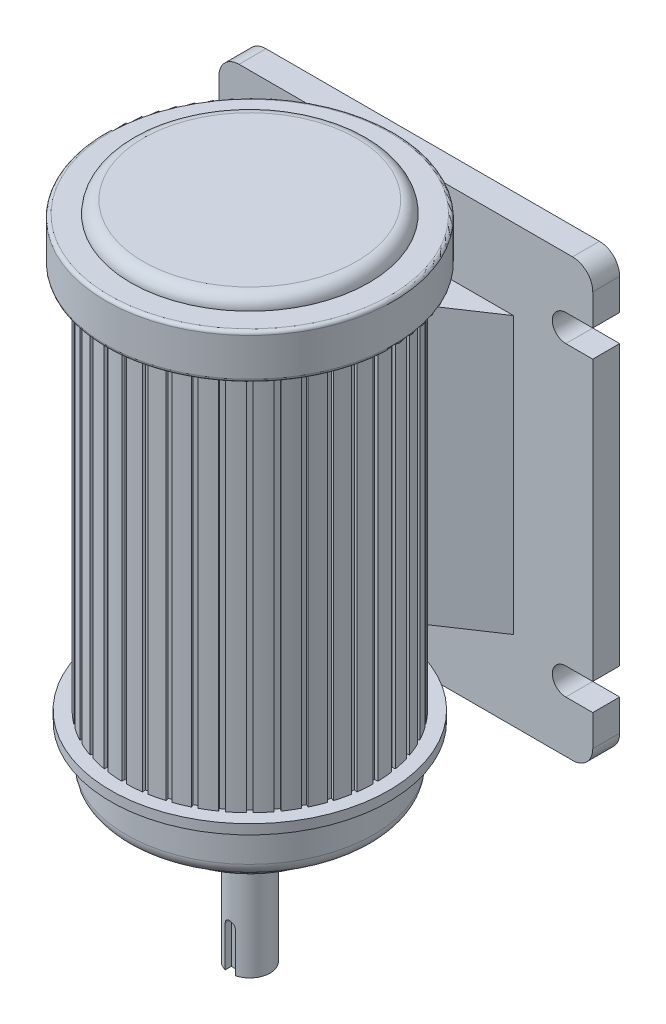
SolidWorks part; units mm, degrees
ref_plane "Front Plane" through (0, 0, 0) normal (0, 0, 1) x (1, 0, 0)
ref_plane "Top Plane" through (0, 0, 0) normal (0, 1, 0) x (1, 0, 0)
ref_plane "Right Plane" through (0, 0, 0) normal (1, 0, 0) x (0, 0, -1)
other "Configuration Table"
sketch "Sketch1" plane through (0, 0, 0) normal (0, 0, 1) x (1, 0, 0)
  line L5 (-18.5243, 142.4072) -> (36.9765, 142.4072)
  line L6 (-18.5243, 142.4072) -> (-18.5243, 77.6701)
  line L7 (-18.5243, 77.6701) -> (36.9765, 77.6701)
  line L12 (36.9765, 142.4072) -> (36.9765, 77.6701)
  line L13 (-18.5243, 142.4072) -> (36.9765, 77.6701) construction
  line L14 (-18.5243, 77.6701) -> (36.9765, 142.4072) construction
  point P2 (9.2261, 110.0386)
extrude "Boss-Extrude1" add sketch "Sketch1" along normal blind 4
sketch "Sketch2" plane through (0, 0, 4) normal (0, 0, 1) x (1, 0, 0)
  line L0 (-14.5271, 134.7549) -> (-18.5243, 134.7549)
  line L1 (-14.5271, 130.7549) -> (-18.5243, 130.7549)
  line L2 (-18.5243, 89.3223) -> (-18.5243, 85.3223)
  line L3 (36.9765, 130.7549) -> (36.9765, 134.7549)
  line L4 (36.9765, 77.6701) -> (36.9765, 142.4072)
  line L5 (36.9765, 142.4072) -> (-18.5243, 142.4072)
  line L6 (-18.5243, 142.4072) -> (-18.5243, 77.6701)
  line L7 (-18.5243, 77.6701) -> (36.9765, 77.6701)
  line L8 (36.9765, 85.3223) -> (36.9765, 89.3223)
  line L10 (-18.5243, 134.7549) -> (-18.5243, 130.7549)
  line L12 (32.9793, 130.7549) -> (36.9765, 130.7549)
  line L13 (32.9793, 134.7549) -> (36.9765, 134.7549)
  line L14 (32.9793, 85.3223) -> (36.9765, 85.3223)
  line L15 (32.9793, 89.3223) -> (36.9765, 89.3223)
  line L16 (-14.5271, 89.3223) -> (-18.5243, 89.3223)
  line L17 (-14.5271, 85.3223) -> (-18.5243, 85.3223)
  arc A0 (-14.5271, 130.7549) -> (-14.5271, 134.7549) centre (-14.5271, 132.7549) ccw
  arc A1 (32.9793, 130.7549) -> (32.9793, 134.7549) centre (32.9793, 132.7549) cw
  arc A2 (32.9793, 89.3223) -> (32.9793, 85.3223) centre (32.9793, 87.3223) ccw
  arc A3 (-14.5271, 89.3223) -> (-14.5271, 85.3223) centre (-14.5271, 87.3223) cw
  dimension "D1" = 0
extrude "Cut-Extrude1" cut sketch "Sketch2" against normal blind 4
fillet "Fillet1" radius 3 4 edges at (36.9765, 142.4072, 2) (-18.5243, 142.4072, 2) (-18.5243, 77.6701, 2) (36.9765, 77.6701, 2)
sketch "Sketch3" plane through (9.2261, -4.2483, 39.612) normal (1, 0, 0) x (0, 1, 0)
  line L0 (114.2869, -35.612) -> (114.2869, 7.7128) construction
  line L1 (93.5706, -35.612) -> (135.0032, -35.612) construction
  line L3 (75.2706, -12.4595) -> (153.1789, -12.4595)
  line L4 (75.2706, -12.4595) -> (75.2706, -0.1704)
  line L5 (87.5845, 6.1907) -> (144.7264, 6.1907)
  line L6 (153.1789, -12.4595) -> (153.1789, 3.3865)
  line L7 (151.3529, 5.2125) -> (151.3529, 8.4086)
  line L8 (150.8529, 8.9086) -> (145.2264, 8.9086)
  line L9 (144.7264, 8.4086) -> (144.7264, 6.1907)
  line L10 (87.5845, 6.1907) -> (87.5845, 8.1927)
  line L11 (87.5845, 8.1927) -> (86.1419, 8.1927)
  line L12 (86.1419, 8.1927) -> (86.1419, 7.166)
  line L13 (86.1419, 7.166) -> (86.1419, 5.8831)
  line L14 (86.1419, 5.8831) -> (80.7228, 5.8831)
  line L15 (78.7228, 3.8831) -> (78.7228, -0.0402)
  line L16 (78.7228, -0.0402) -> (77.8437, -0.6822)
  line L17 (77.8437, -0.6822) -> (77.8437, 0.7371)
  line L18 (77.6437, 0.9371) -> (76.7521, 0.9371)
  line L19 (76.5521, 0.7371) -> (76.5521, 0.0296)
  line L20 (76.5521, 0.0296) -> (75.4706, 0.0296)
  arc A0 (153.1789, 3.3865) -> (151.3529, 5.2125) centre (151.3529, 3.3865) ccw
  arc A1 (145.2264, 8.9086) -> (144.7264, 8.4086) centre (145.2264, 8.4086) ccw
  arc A2 (151.3529, 8.4086) -> (150.8529, 8.9086) centre (150.8529, 8.4086) ccw
  arc A3 (80.7228, 5.8831) -> (78.7228, 3.8831) centre (80.7228, 3.8831) ccw
  arc A4 (76.7521, 0.9371) -> (76.5521, 0.7371) centre (76.7521, 0.7371) ccw
  arc A5 (77.8437, 0.7371) -> (77.6437, 0.9371) centre (77.6437, 0.7371) ccw
  arc A6 (75.4706, 0.0296) -> (75.2706, -0.1704) centre (75.4706, -0.1704) ccw
  dimension "D1" = 0.5
  dimension "D2" = 2
  dimension "D3" = 0.2
  dimension "D4" = 0.2
revolve "Revolve1" add sketch "Sketch3" angle 360 about L3
ref_plane "Plane1" through (0, 109.9765, 0) normal (0, 1, 0) x (1, 0, 0)
sketch "Sketch5" plane through (0, 83.3362, 0) normal (0, 1, 0) x (1, 0, 0)
  line L0 (11.7885, -8.6793) -> (11.7149, -9.1436)
  line L6 (8.8671, -8.5059) -> (8.8671, -8.976)
  line L7 (8.8671, -8.976) -> (9.5851, -8.976)
  line L8 (9.5851, -8.5059) -> (9.5851, -8.976)
  line L9 (9.2261, -8.5024) -> (9.5851, -8.976) construction
  line L10 (8.8671, -8.976) -> (9.2261, -8.5024) construction
  line L11 (11.7149, -9.1436) -> (12.4241, -9.2559)
  line L12 (12.4977, -8.7916) -> (12.4241, -9.2559)
  line L13 (12.1436, -8.732) -> (12.4241, -9.2559) construction
  line L14 (11.7149, -9.1436) -> (12.1436, -8.732) construction
  line L15 (14.6468, -9.3075) -> (14.5015, -9.7546)
  line L16 (14.5015, -9.7546) -> (15.1844, -9.9765)
  line L17 (15.3297, -9.5294) -> (15.1844, -9.9765)
  line L18 (14.9893, -9.4152) -> (15.1844, -9.9765) construction
  line L19 (14.5015, -9.7546) -> (14.9893, -9.4152) construction
  line L20 (17.3716, -10.3752) -> (17.1582, -10.7941)
  line L21 (17.1582, -10.7941) -> (17.798, -11.1201)
  line L22 (18.0114, -10.7012) -> (17.798, -11.1201)
  line L23 (17.6931, -10.5351) -> (17.798, -11.1201) construction
  line L24 (17.1582, -10.7941) -> (17.6931, -10.5351) construction
  line L25 (19.8959, -11.856) -> (19.6196, -12.2364)
  line L26 (19.6196, -12.2364) -> (20.2005, -12.6584)
  line L27 (20.4768, -12.2781) -> (20.2005, -12.6584)
  line L28 (20.1884, -12.0643) -> (20.2005, -12.6584) construction
  line L29 (19.6196, -12.2364) -> (20.1884, -12.0643) construction
  line L30 (22.1574, -13.7135) -> (21.825, -14.0459)
  line L31 (21.825, -14.0459) -> (22.3327, -14.5536)
  line L32 (22.6652, -14.2212) -> (22.3327, -14.5536)
  line L33 (22.4137, -13.9649) -> (22.3327, -14.5536) construction
  line L34 (21.825, -14.0459) -> (22.4137, -13.9649) construction
  line L35 (24.1006, -15.9018) -> (23.7202, -16.1782)
  line L36 (23.7202, -16.1782) -> (24.1423, -16.7591)
  line L37 (24.5226, -16.4827) -> (24.1423, -16.7591)
  line L38 (24.3144, -16.1903) -> (24.1423, -16.7591) construction
  line L39 (23.7202, -16.1782) -> (24.3144, -16.1903) construction
  line L40 (25.6774, -18.3672) -> (25.2586, -18.5807)
  line L41 (25.2586, -18.5807) -> (25.5845, -19.2204)
  line L42 (26.0034, -19.007) -> (25.5845, -19.2204)
  line L43 (25.8435, -18.6856) -> (25.5845, -19.2204) construction
  line L44 (25.2586, -18.5807) -> (25.8435, -18.6856) construction
  line L45 (26.8492, -21.049) -> (26.4021, -21.1942)
  line L46 (26.4021, -21.1942) -> (26.624, -21.8771)
  line L47 (27.0711, -21.7319) -> (26.624, -21.8771)
  line L48 (26.9634, -21.3893) -> (26.624, -21.8771) construction
  line L49 (26.4021, -21.1942) -> (26.9634, -21.3893) construction
  line L50 (27.587, -23.881) -> (27.1227, -23.9545)
  line L51 (27.1227, -23.9545) -> (27.2351, -24.6637)
  line L52 (27.6994, -24.5902) -> (27.2351, -24.6637)
  line L53 (27.6466, -24.235) -> (27.2351, -24.6637) construction
  line L54 (27.1227, -23.9545) -> (27.6466, -24.235) construction
  line L55 (27.8728, -26.7935) -> (27.4027, -26.7935)
  line L56 (27.4027, -26.7935) -> (27.4027, -27.5116)
  line L57 (27.8728, -27.5116) -> (27.4027, -27.5116)
  line L58 (27.8762, -27.1526) -> (27.4027, -27.5116) construction
  line L59 (27.4027, -26.7935) -> (27.8762, -27.1526) construction
  line L60 (27.6994, -29.7149) -> (27.2351, -29.6414)
  line L61 (27.2351, -29.6414) -> (27.1227, -30.3506)
  line L62 (27.587, -30.4241) -> (27.1227, -30.3506)
  line L63 (27.6466, -30.0701) -> (27.1227, -30.3506) construction
  line L64 (27.2351, -29.6414) -> (27.6466, -30.0701) construction
  line L65 (27.0711, -32.5733) -> (26.624, -32.428)
  line L66 (26.624, -32.428) -> (26.4021, -33.1109)
  line L67 (26.8492, -33.2561) -> (26.4021, -33.1109)
  line L68 (26.9634, -32.9158) -> (26.4021, -33.1109) construction
  line L69 (26.624, -32.428) -> (26.9634, -32.9158) construction
  line L70 (26.0034, -35.2981) -> (25.5845, -35.0847)
  line L71 (25.5845, -35.0847) -> (25.2586, -35.7244)
  line L72 (25.6774, -35.9379) -> (25.2586, -35.7244)
  line L73 (25.8435, -35.6195) -> (25.2586, -35.7244) construction
  line L74 (25.5845, -35.0847) -> (25.8435, -35.6195) construction
  line L75 (24.5226, -37.8224) -> (24.1423, -37.546)
  line L76 (24.1423, -37.546) -> (23.7202, -38.1269)
  line L77 (24.1006, -38.4033) -> (23.7202, -38.1269)
  line L78 (24.3144, -38.1148) -> (23.7202, -38.1269) construction
  line L79 (24.1423, -37.546) -> (24.3144, -38.1148) construction
  line L80 (22.6652, -40.0839) -> (22.3327, -39.7515)
  line L81 (22.3327, -39.7515) -> (21.825, -40.2592)
  line L82 (22.1574, -40.5916) -> (21.825, -40.2592)
  line L83 (22.4137, -40.3402) -> (21.825, -40.2592) construction
  line L84 (22.3327, -39.7515) -> (22.4137, -40.3402) construction
  line L85 (20.4768, -42.027) -> (20.2005, -41.6467)
  line L86 (20.2005, -41.6467) -> (19.6196, -42.0688)
  line L87 (19.8959, -42.4491) -> (19.6196, -42.0688)
  line L88 (20.1884, -42.2408) -> (19.6196, -42.0688) construction
  line L89 (20.2005, -41.6467) -> (20.1884, -42.2408) construction
  line L90 (18.0114, -43.6039) -> (17.798, -43.185)
  line L91 (17.798, -43.185) -> (17.1582, -43.511)
  line L92 (17.3716, -43.9299) -> (17.1582, -43.511)
  line L93 (17.6931, -43.77) -> (17.1582, -43.511) construction
  line L94 (17.798, -43.185) -> (17.6931, -43.77) construction
  line L95 (15.3297, -44.7757) -> (15.1844, -44.3286)
  line L96 (15.1844, -44.3286) -> (14.5015, -44.5505)
  line L97 (14.6468, -44.9976) -> (14.5015, -44.5505)
  line L98 (14.9893, -44.8899) -> (14.5015, -44.5505) construction
  line L99 (15.1844, -44.3286) -> (14.9893, -44.8899) construction
  line L100 (12.4977, -45.5135) -> (12.4241, -45.0492)
  line L101 (12.4241, -45.0492) -> (11.7149, -45.1615)
  line L102 (11.7885, -45.6258) -> (11.7149, -45.1615)
  line L103 (12.1436, -45.5731) -> (11.7149, -45.1615) construction
  line L104 (12.4241, -45.0492) -> (12.1436, -45.5731) construction
  line L105 (9.5851, -45.7992) -> (9.5851, -45.3292)
  line L106 (9.5851, -45.3292) -> (8.8671, -45.3292)
  line L107 (8.8671, -45.7992) -> (8.8671, -45.3292)
  line L108 (9.2261, -45.8027) -> (8.8671, -45.3292) construction
  line L109 (9.5851, -45.3292) -> (9.2261, -45.8027) construction
  line L110 (6.6637, -45.6258) -> (6.7372, -45.1615)
  line L111 (6.7372, -45.1615) -> (6.028, -45.0492)
  line L112 (5.9545, -45.5135) -> (6.028, -45.0492)
  line L113 (6.3086, -45.5731) -> (6.028, -45.0492) construction
  line L114 (6.7372, -45.1615) -> (6.3086, -45.5731) construction
  line L115 (3.8054, -44.9976) -> (3.9506, -44.5505)
  line L116 (3.9506, -44.5505) -> (3.2678, -44.3286)
  line L117 (3.1225, -44.7757) -> (3.2678, -44.3286)
  line L118 (3.4629, -44.8899) -> (3.2678, -44.3286) construction
  line L119 (3.9506, -44.5505) -> (3.4629, -44.8899) construction
  line L120 (1.0805, -43.9299) -> (1.294, -43.511)
  line L121 (1.294, -43.511) -> (0.6542, -43.185)
  line L122 (0.4408, -43.6039) -> (0.6542, -43.185)
  line L123 (0.7591, -43.77) -> (0.6542, -43.185) construction
  line L124 (1.294, -43.511) -> (0.7591, -43.77) construction
  line L125 (-1.4437, -42.4491) -> (-1.1674, -42.0688)
  line L126 (-1.1674, -42.0688) -> (-1.7483, -41.6467)
  line L127 (-2.0246, -42.027) -> (-1.7483, -41.6467)
  line L128 (-1.7362, -42.2408) -> (-1.7483, -41.6467) construction
  line L129 (-1.1674, -42.0688) -> (-1.7362, -42.2408) construction
  line L130 (-3.7053, -40.5916) -> (-3.3729, -40.2592)
  line L131 (-3.3729, -40.2592) -> (-3.8806, -39.7515)
  line L132 (-4.213, -40.0839) -> (-3.8806, -39.7515)
  line L133 (-3.9616, -40.3402) -> (-3.8806, -39.7515) construction
  line L134 (-3.3729, -40.2592) -> (-3.9616, -40.3402) construction
  line L135 (-5.6484, -38.4033) -> (-5.2681, -38.1269)
  line L136 (-5.2681, -38.1269) -> (-5.6901, -37.546)
  line L137 (-6.0704, -37.8224) -> (-5.6901, -37.546)
  line L138 (-5.8622, -38.1148) -> (-5.6901, -37.546) construction
  line L139 (-5.2681, -38.1269) -> (-5.8622, -38.1148) construction
  line L140 (-7.2253, -35.9379) -> (-6.8064, -35.7244)
  line L141 (-6.8064, -35.7244) -> (-7.1324, -35.0847)
  line L142 (-7.5512, -35.2981) -> (-7.1324, -35.0847)
  line L143 (-7.3913, -35.6195) -> (-7.1324, -35.0847) construction
  line L144 (-6.8064, -35.7244) -> (-7.3913, -35.6195) construction
  line L145 (-8.397, -33.2561) -> (-7.9499, -33.1109)
  line L146 (-7.9499, -33.1109) -> (-8.1718, -32.428)
  line L147 (-8.6189, -32.5733) -> (-8.1718, -32.428)
  line L148 (-8.5113, -32.9158) -> (-8.1718, -32.428) construction
  line L149 (-7.9499, -33.1109) -> (-8.5113, -32.9158) construction
  line L150 (-9.1349, -30.4241) -> (-8.6706, -30.3506)
  line L151 (-8.6706, -30.3506) -> (-8.7829, -29.6414)
  line L152 (-9.2472, -29.7149) -> (-8.7829, -29.6414)
  line L153 (-9.1945, -30.0701) -> (-8.7829, -29.6414) construction
  line L154 (-8.6706, -30.3506) -> (-9.1945, -30.0701) construction
  line L155 (-9.4206, -27.5116) -> (-8.9505, -27.5116)
  line L156 (-8.9505, -27.5116) -> (-8.9505, -26.7935)
  line L157 (-9.4206, -26.7935) -> (-8.9505, -26.7935)
  line L158 (-9.4241, -27.1526) -> (-8.9505, -26.7935) construction
  line L159 (-8.9505, -27.5116) -> (-9.4241, -27.1526) construction
  line L160 (-9.2472, -24.5902) -> (-8.7829, -24.6637)
  line L161 (-8.7829, -24.6637) -> (-8.6706, -23.9545)
  line L162 (-9.1349, -23.881) -> (-8.6706, -23.9545)
  line L163 (-9.1945, -24.235) -> (-8.6706, -23.9545) construction
  line L164 (-8.7829, -24.6637) -> (-9.1945, -24.235) construction
  line L165 (-8.6189, -21.7319) -> (-8.1718, -21.8771)
  line L166 (-8.1718, -21.8771) -> (-7.9499, -21.1942)
  line L167 (-8.397, -21.049) -> (-7.9499, -21.1942)
  line L168 (-8.5113, -21.3893) -> (-7.9499, -21.1942) construction
  line L169 (-8.1718, -21.8771) -> (-8.5113, -21.3893) construction
  line L170 (-7.5512, -19.007) -> (-7.1324, -19.2204)
  line L171 (-7.1324, -19.2204) -> (-6.8064, -18.5807)
  line L172 (-7.2253, -18.3672) -> (-6.8064, -18.5807)
  line L173 (-7.3913, -18.6856) -> (-6.8064, -18.5807) construction
  line L174 (-7.1324, -19.2204) -> (-7.3913, -18.6856) construction
  line L175 (-6.0704, -16.4827) -> (-5.6901, -16.7591)
  line L176 (-5.6901, -16.7591) -> (-5.2681, -16.1782)
  line L177 (-5.6484, -15.9018) -> (-5.2681, -16.1782)
  line L178 (-5.8622, -16.1903) -> (-5.2681, -16.1782) construction
  line L179 (-5.6901, -16.7591) -> (-5.8622, -16.1903) construction
  line L180 (-4.213, -14.2212) -> (-3.8806, -14.5536)
  line L181 (-3.8806, -14.5536) -> (-3.3729, -14.0459)
  line L182 (-3.7053, -13.7135) -> (-3.3729, -14.0459)
  line L183 (-3.9616, -13.9649) -> (-3.3729, -14.0459) construction
  line L184 (-3.8806, -14.5536) -> (-3.9616, -13.9649) construction
  line L185 (-2.0246, -12.2781) -> (-1.7483, -12.6584)
  line L186 (-1.7483, -12.6584) -> (-1.1674, -12.2364)
  line L187 (-1.4437, -11.856) -> (-1.1674, -12.2364)
  line L188 (-1.7362, -12.0643) -> (-1.1674, -12.2364) construction
  line L189 (-1.7483, -12.6584) -> (-1.7362, -12.0643) construction
  line L190 (0.4408, -10.7012) -> (0.6542, -11.1201)
  line L191 (0.6542, -11.1201) -> (1.294, -10.7941)
  line L192 (1.0805, -10.3752) -> (1.294, -10.7941)
  line L193 (0.7591, -10.5351) -> (1.294, -10.7941) construction
  line L194 (0.6542, -11.1201) -> (0.7591, -10.5351) construction
  line L195 (3.1225, -9.5294) -> (3.2678, -9.9765)
  line L196 (3.2678, -9.9765) -> (3.9506, -9.7546)
  line L197 (3.8054, -9.3075) -> (3.9506, -9.7546)
  line L198 (3.4629, -9.4152) -> (3.9506, -9.7546) construction
  line L199 (3.2678, -9.9765) -> (3.4629, -9.4152) construction
  line L200 (5.9545, -8.7916) -> (6.028, -9.2559)
  line L201 (6.028, -9.2559) -> (6.7372, -9.1436)
  line L202 (6.6637, -8.6793) -> (6.7372, -9.1436)
  line L203 (6.3086, -8.732) -> (6.7372, -9.1436) construction
  line L204 (6.028, -9.2559) -> (6.3086, -8.732) construction
  circle A0 centre (9.2261, -27.1526) radius 18.6502 construction
  arc A1 (12.4977, -8.7916) -> (11.7885, -8.6793) centre (9.2261, -27.1526) ccw
  arc A3 (9.5851, -8.5059) -> (8.8671, -8.5059) centre (9.2261, -27.1526) ccw
  arc A4 (15.3297, -9.5294) -> (14.6468, -9.3075) centre (9.2261, -27.1526) ccw
  arc A5 (18.0114, -10.7012) -> (17.3716, -10.3752) centre (9.2261, -27.1526) ccw
  arc A6 (20.4768, -12.2781) -> (19.8959, -11.856) centre (9.2261, -27.1526) ccw
  arc A7 (22.6652, -14.2212) -> (22.1574, -13.7135) centre (9.2261, -27.1526) ccw
  arc A8 (24.5226, -16.4827) -> (24.1006, -15.9018) centre (9.2261, -27.1526) ccw
  arc A9 (26.0034, -19.007) -> (25.6774, -18.3672) centre (9.2261, -27.1526) ccw
  arc A10 (27.0711, -21.7319) -> (26.8492, -21.049) centre (9.2261, -27.1526) ccw
  arc A11 (27.6994, -24.5902) -> (27.587, -23.881) centre (9.2261, -27.1526) ccw
  arc A12 (27.8728, -27.5116) -> (27.8728, -26.7935) centre (9.2261, -27.1526) ccw
  arc A13 (27.587, -30.4241) -> (27.6994, -29.7149) centre (9.2261, -27.1526) ccw
  arc A14 (26.8492, -33.2561) -> (27.0711, -32.5733) centre (9.2261, -27.1526) ccw
  arc A15 (25.6774, -35.9379) -> (26.0034, -35.2981) centre (9.2261, -27.1526) ccw
  arc A16 (24.1006, -38.4033) -> (24.5226, -37.8224) centre (9.2261, -27.1526) ccw
  arc A17 (22.1574, -40.5916) -> (22.6652, -40.0839) centre (9.2261, -27.1526) ccw
  arc A18 (19.8959, -42.4491) -> (20.4768, -42.027) centre (9.2261, -27.1526) ccw
  arc A19 (17.3716, -43.9299) -> (18.0114, -43.6039) centre (9.2261, -27.1526) ccw
  arc A20 (14.6468, -44.9976) -> (15.3297, -44.7757) centre (9.2261, -27.1526) ccw
  arc A21 (11.7885, -45.6258) -> (12.4977, -45.5135) centre (9.2261, -27.1526) ccw
  arc A22 (8.8671, -45.7992) -> (9.5851, -45.7992) centre (9.2261, -27.1526) ccw
  arc A23 (5.9545, -45.5135) -> (6.6637, -45.6258) centre (9.2261, -27.1526) ccw
  arc A24 (3.1225, -44.7757) -> (3.8054, -44.9976) centre (9.2261, -27.1526) ccw
  arc A25 (0.4408, -43.6039) -> (1.0805, -43.9299) centre (9.2261, -27.1526) ccw
  arc A26 (-2.0246, -42.027) -> (-1.4437, -42.4491) centre (9.2261, -27.1526) ccw
  arc A27 (-4.213, -40.0839) -> (-3.7053, -40.5916) centre (9.2261, -27.1526) ccw
  arc A28 (-6.0704, -37.8224) -> (-5.6484, -38.4033) centre (9.2261, -27.1526) ccw
  arc A29 (-7.5512, -35.2981) -> (-7.2253, -35.9379) centre (9.2261, -27.1526) ccw
  arc A30 (-8.6189, -32.5733) -> (-8.397, -33.2561) centre (9.2261, -27.1526) ccw
  arc A31 (-9.2472, -29.7149) -> (-9.1349, -30.4241) centre (9.2261, -27.1526) ccw
  arc A32 (-9.4206, -26.7935) -> (-9.4206, -27.5116) centre (9.2261, -27.1526) ccw
  arc A33 (-9.1349, -23.881) -> (-9.2472, -24.5902) centre (9.2261, -27.1526) ccw
  arc A34 (-8.397, -21.049) -> (-8.6189, -21.7319) centre (9.2261, -27.1526) ccw
  arc A35 (-7.2253, -18.3672) -> (-7.5512, -19.007) centre (9.2261, -27.1526) ccw
  arc A36 (-5.6484, -15.9018) -> (-6.0704, -16.4827) centre (9.2261, -27.1526) ccw
  arc A37 (-3.7053, -13.7135) -> (-4.213, -14.2212) centre (9.2261, -27.1526) ccw
  arc A38 (-1.4437, -11.856) -> (-2.0246, -12.2781) centre (9.2261, -27.1526) ccw
  arc A39 (1.0805, -10.3752) -> (0.4408, -10.7012) centre (9.2261, -27.1526) ccw
  arc A40 (3.8054, -9.3075) -> (3.1225, -9.5294) centre (9.2261, -27.1526) ccw
  arc A41 (6.6637, -8.6793) -> (5.9545, -8.7916) centre (9.2261, -27.1526) ccw
  point P5 (9.2261, -8.5024)
  point P7 (12.1436, -8.732)
  point P17 (14.9893, -9.4152)
  point P23 (17.6931, -10.5351)
  point P29 (20.1884, -12.0643)
  point P35 (22.4137, -13.9649)
  point P41 (24.3144, -16.1903)
  point P47 (25.8435, -18.6856)
  point P53 (26.9634, -21.3893)
  point P59 (27.6466, -24.235)
  point P65 (27.8762, -27.1526)
  point P71 (27.6466, -30.0701)
  point P77 (26.9634, -32.9158)
  point P83 (25.8435, -35.6195)
  point P89 (24.3144, -38.1148)
  point P95 (22.4137, -40.3402)
  point P101 (20.1884, -42.2408)
  point P107 (17.6931, -43.77)
  point P113 (14.9893, -44.8899)
  point P119 (12.1436, -45.5731)
  point P125 (9.2261, -45.8027)
  point P131 (6.3086, -45.5731)
  point P137 (3.4629, -44.8899)
  point P143 (0.7591, -43.77)
  point P149 (-1.7362, -42.2408)
  point P155 (-3.9616, -40.3402)
  point P161 (-5.8622, -38.1148)
  point P167 (-7.3913, -35.6195)
  point P173 (-8.5113, -32.9158)
  point P179 (-9.1945, -30.0701)
  point P185 (-9.4241, -27.1526)
  point P191 (-9.1945, -24.235)
  point P197 (-8.5113, -21.3893)
  point P203 (-7.3913, -18.6856)
  point P209 (-5.8622, -16.1903)
  point P215 (-3.9616, -13.9649)
  point P221 (-1.7362, -12.0643)
  point P227 (0.7591, -10.5351)
  point P233 (3.4629, -9.4152)
  point P239 (6.3086, -8.732)
  point P245 (9.2261, -27.1526)
  dimension "D1" = 40
extrude "Cut-Extrude2" cut sketch "Sketch5" along normal up to surface (57.1419 mm away) up to face at (9.2261, 140.4781, 8.5024)
sketch "Sketch6" plane through (0, 109.9765, 0) normal (0, 1, 0) x (1, 0, 0)
  line L0 (-6.7709, -4) -> (9.2261, -14.7109)
  line L1 (33.9765, -4) -> (-15.5243, -4) construction
  line L3 (25.2231, -4) -> (-6.7709, -4)
  line L4 (25.2231, -4) -> (9.2261, -14.7109)
extrude "Boss-Extrude2" add sketch "Sketch6" along normal mid plane 41
sketch "Sketch7" plane through (0, 71.0224, 0) normal (0, -1, 0) x (1, 0, 0)
  circle A0 centre (9.2261, 27.1526) radius 4.5336
  circle A1 centre (9.2261, 27.1526) radius 3.9511
extrude "Boss-Extrude3" add sketch "Sketch7" along normal mid plane 1
sketch "Sketch8" plane through (0, 71.0224, 0) normal (0, -1, 0) x (1, 0, 0)
  circle A0 centre (9.2261, 27.1526) radius 3
extrude "Boss-Extrude4" add sketch "Sketch8" along normal blind 20
sketch "Sketch9" plane through (0, 51.0224, 0) normal (0, -1, 0) x (1, 0, 0)
  line L1 (8.4761, 31.1526) -> (9.9761, 31.1526)
  line L2 (8.4761, 31.1526) -> (8.4761, 29.1526)
  line L3 (8.4761, 29.1526) -> (9.9761, 29.1526)
  line L4 (9.9761, 31.1526) -> (9.9761, 29.1526)
  line L5 (8.4761, 31.1526) -> (9.9761, 29.1526) construction
  line L6 (8.4761, 29.1526) -> (9.9761, 31.1526) construction
  circle A0 centre (9.2261, 27.1526) radius 3 construction
  circle A1 centre (9.2261, 27.1526) radius 3 construction
  point P0 (9.2261, 30.1526)
extrude "Cut-Extrude3" cut sketch "Sketch9" against normal blind 6
sketch "Sketch10" plane through (0, 0, 29.1526) normal (0, 0, 1) x (1, 0, 0)
  line L0 (8.4761, 57.0224) -> (9.9761, 57.0224) construction
  circle A0 centre (9.2261, 57.0224) radius 0.75
extrude "Cut-Extrude4" cut sketch "Sketch10" along normal blind 2
